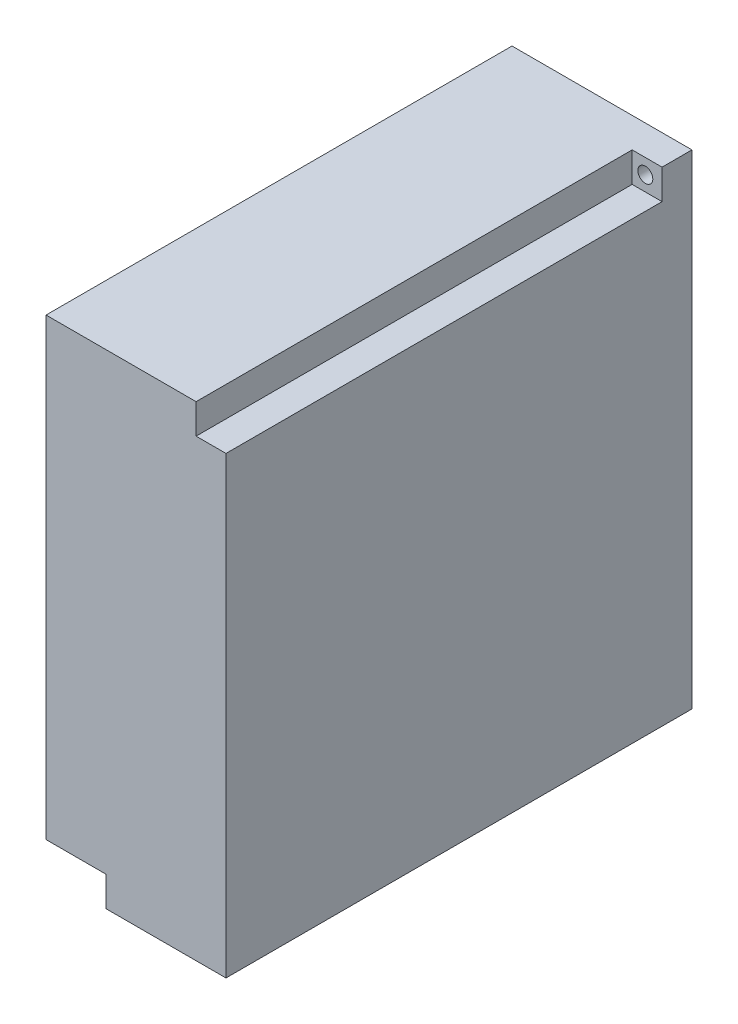
from build123d import *

# Parameters (mm, degrees)
SKETCH1_W          = 60.2
SKETCH1_H          = 162
EXTRUDE1_DEPTH     = 155.9
SKETCH2_W          = 20
SKETCH2_H          = 10
SKETCH2_W_2        = 10
CUT_EXTRUDE1_DEPTH = 145.9
SKETCH3_R          = 2.5
CUT_EXTRUDE2_DEPTH = 179.246514692


with BuildPart() as part:
    # Sketch1 → Extrude1 (new body)
    with BuildSketch(Plane.XY):
        Rectangle(SKETCH1_W, SKETCH1_H)
    extrude(amount=EXTRUDE1_DEPTH)

    # Sketch2 → Cut-Extrude1 (cut)
    with BuildSketch(Plane.XY.offset(155.9)):
        with Locations((-20.1, -76)):
            Rectangle(SKETCH2_W, SKETCH2_H)
        with Locations((25.1, 76)):
            Rectangle(SKETCH2_W_2, SKETCH2_H)
    extrude(amount=-CUT_EXTRUDE1_DEPTH, mode=Mode.SUBTRACT)

    # Sketch3 → Cut-Extrude2 (cut, through all)
    with BuildSketch(Plane.XY.offset(155.9)):
        with Locations((24.5, 76)):
            Circle(SKETCH3_R)
        with Locations((-24.5, -76)):
            Circle(SKETCH3_R)
    extrude(amount=-CUT_EXTRUDE2_DEPTH, mode=Mode.SUBTRACT)


solid = part.part
